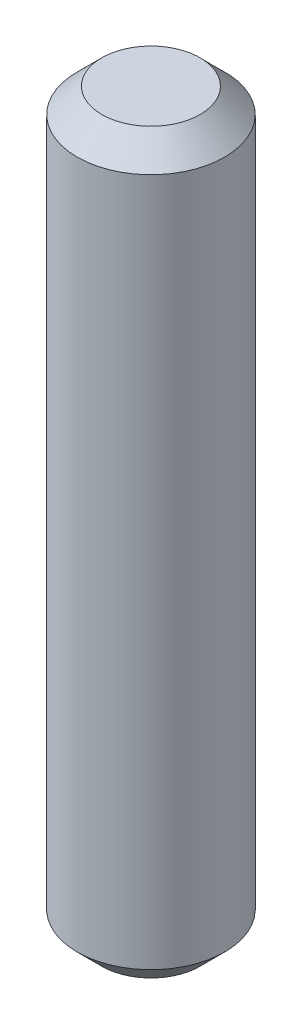
SolidWorks part; units mm, degrees
ref_plane "Front Plane" through (0, 0, 0) normal (0, 0, 1) x (1, 0, 0)
ref_plane "Top Plane" through (0, 0, 0) normal (0, 1, 0) x (1, 0, 0)
ref_plane "Right Plane" through (0, 0, 0) normal (1, 0, 0) x (0, 0, -1)
other "Configuration Table"
sketch "Sketch1" plane through (0, 0, 0) normal (0, 1, 0) x (1, 0, 0)
  circle A0 centre (0, 0) radius 1.5
  dimension "D1" = 3
extrude "Boss-Extrude1" add sketch "Sketch1" along normal blind 15
chamfer "Chamfer1" distance 0.5 2 edges at (0, 0, 1.5) (0, 15, 1.5)
